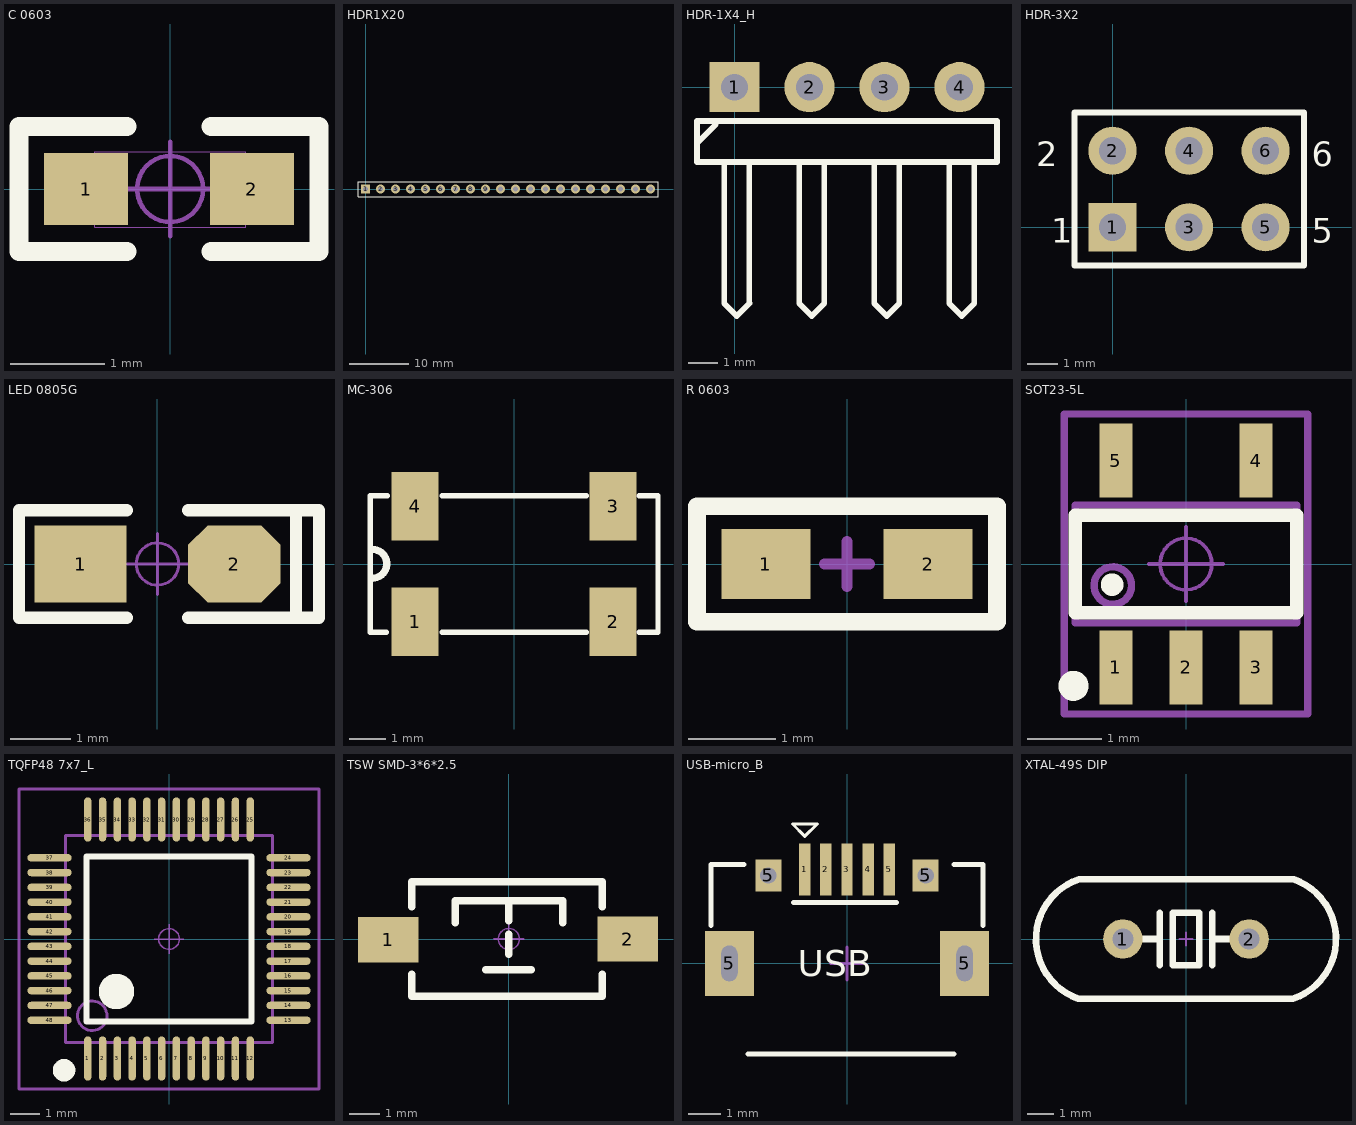
[diagram p0: the footprints below, top view; thin cyan lines are the x and y axes]
# Altium footprint library MISC82227-4.PcbLib: 12 footprints
Each footprint in its own frame and in the unit in brackets; x right, y up, seen from the top. Pads: shape width x height; smd on the part's side, far side on the other; paste and mask are expansions set on the pad; w line width, h text height; cw(c..) or ccw(c..) is an arc to the next point about the centre after c.

## C 0603 [mil] "Non-polarised SMD capacitor"
pads (2):
  rect 35x30 smd: 1(-35,0) 2(34,0)
Top Overlay:
  lines w8: -18,-26 -63,-26 -63,26 -18,26 ; 17,-26 62,-26 62,26 17,26
Mechanical 13:
  lines w0.39: -31.5,-16 31.5,-16 31.5,15.5 -31.5,15.5 -31.5,-16
Mechanical 15:
  circle w1.97: c0,0 r13.78
  lines w1.97: -19.68,0 19.68,0 ; 0,-19.68 0,19.68
3D body "C 0603.STEP": height 31.89, standoff -0.39, extent -31.5,-16.14 31.5,16.14

## HDR1X20 [mm] "Connector; Header; 20 Position"
height 4.32
pads (20):
  rect 1.5x1.5 hole 0.9: 1(0,0)
  round 1.5 hole 0.9: 2(2.54,0) 3(5.08,0) 4(7.62,0) 5(10.16,0) 6(12.7,0) 7(15.24,0) 8(17.78,0) 9(20.32,0) 10(22.86,0) 11(25.4,0) 12(27.94,0) 13(30.48,0) 14(33.02,0) 15(35.56,0) 16(38.1,0) 17(40.64,0) 18(43.18,0) 19(45.72,0) 20(48.26,0)
Top Overlay:
  lines w0.2: -1.27,-1.27 49.53,-1.27 49.53,1.27 0.635,1.27 -1.27,1.27 -1.27,-1.27

## HDR-1X4_H [mm] "Right-angle pin header, 4 pins"
pads (4):
  rect 1.7x1.7 hole 0.9: 1(0,0)
  round 1.7 hole 0.9: 2(2.54,0) 3(5.08,0) 4(7.62,0)
Top Overlay:
  lines w0.2: -1.27,-1.905 -0.635,-1.27 ; -0.348,-2.54 -0.348,-7.332 0.075,-7.755 0.499,-7.332 0.508,-7.323 ; 0.499,-7.323 0.499,-2.54 ; 2.192,-2.54 2.192,-7.332 2.615,-7.755 3.039,-7.332 ; 3.039,-7.323 3.039,-2.54 ; 4.732,-2.54 4.732,-7.332 5.155,-7.755 5.579,-7.332 ; 5.579,-7.323 5.579,-2.54 ; 7.272,-2.54 7.272,-7.332 7.695,-7.755 8.119,-7.332 ; 8.119,-7.323 8.119,-2.54 ; -1.27,-2.54 8.89,-2.54 8.89,-1.143 0.508,-1.143 -1.27,-1.143 -1.27,-2.54
3D body "HDR2.54-1P_H.STEP": height 4.85, standoff -3, extent 6.35,-7.77 8.89,1.27
3D body "HDR2.54-1P_H.STEP": height 4.85, standoff -3, extent 3.81,-7.77 6.35,1.27
3D body "HDR2.54-1P_H.STEP": height 4.85, standoff -3, extent 1.27,-7.77 3.81,1.27
3D body "HDR2.54-1P_H.STEP": height 4.85, standoff -3, extent -1.27,-7.77 1.27,1.27

## HDR-3X2 [mm] "Dual-row pin header, 3x2 pins"
pads (6):
  rect 1.6x1.6 hole 0.9: 1(0,0)
  round 1.6 hole 0.9: 2(0,2.54) 3(2.54,0) 4(2.54,2.54) 5(5.08,0) 6(5.08,2.54)
Top Overlay:
  lines w0.2: 1.482,-1.27 6.35,-1.27 ; 6.35,-1.27 6.35,3.81 -1.27,3.81 -1.27,-1.27 6.35,-1.27
  text "6" at 6.604,2.032 h0.81
  text "5" at 6.604,-0.508 h0.81
  text "2" at -2.54,2.032 h0.81
  text "1" at -2.032,-0.508 h0.81
3D body "HDR2.54-1x2P.STEP": height 8.5, standoff -3, extent 3.81,-1.27 6.35,3.81
3D body "HDR2.54-1x2P.STEP": height 8.5, standoff -3, extent -1.27,-1.27 1.27,3.81
3D body "HDR2.54-1x2P.STEP": height 8.5, standoff -3, extent 1.27,-1.27 3.81,3.81

## LED 0805G [mil] "Green 0805LED"
pads (2):
  rect 60x50 smd: 1(-50,0)
  oct 60x50 smd: 2(50,0)
Top Overlay:
  lines w8: -20,-35 -90,-35 -90,35 -20,35 ; 20,-35 105,-35 105,35 20,35 ; 90,-35 90,35
Mechanical 15:
  circle w1.97: c0,0 r13.78
  lines w1.97: -19.68,0 19.68,0 ; 0,-19.68 0,19.68
3D body "LED 0805玻璃罩.STEP": height 31.69, standoff 12.01, extent -29.49,-24.65 29.49,24.65
3D body "LED 0805-G.STEP": height 26.33, standoff -0.16, extent -39.37,-24.65 39.37,24.65

## MC-306 [mm]
height 1.6
pads (4):
  rect 1.3x1.9 smd: 1(-2.75,-1.6) 2(2.75,-1.6) 3(2.75,1.6) 4(-2.75,1.6)
Top Overlay:
  lines w0.152: -3.556,-1.9 -4,-1.9 -4,1.9 -3.531,1.9 ; -2,-1.9 2,-1.9 ; -2,1.9 2,1.9 ; 3.48,-1.9 4,-1.9 4,1.9 3.48,1.9
  lines w0.2: -3.937,-0.394 ccw(c-3.937,0.006) -3.937,0.406

## R 0603 [mil] "1/10W SMD resistor"
pads (2):
  rect 40x31.5 smd: 1(-36.5,0) 2(36.5,0)
Top Overlay:
  lines w8: -67.5,-26 -67.5,26 67.5,26 67.5,-26 -67.5,-26
Mechanical 15:
  lines w5: -10,0 10,0 ; 0,-10 0,10
3D body "R 0603.STEP": height 15.79, standoff -0.13, extent -31.5,-15.75 31.5,15.75

## SOT23-5L [mm] "3x1.6x1.1mm (LxWxH)"
pads (5):
  rect 0.45x1 smd: 1(-0.95,-1.4) 2(0,-1.4) 3(0.95,-1.4) 4(0.95,1.4) 5(-0.95,1.4)
Top Overlay:
  circle w0.254: c-1.524,-1.651 r0.076
  circle w0.254: c-1.001,-0.279 r0.025
  lines w0.178: -1.5,-0.66 -1.5,0.66 1.5,0.66 1.5,-0.66 -1.5,-0.66
Mechanical 13:
  circle w0.1: c-0.992,-0.292 r0.254
  lines w0.1: -1.5,-0.8 1.5,-0.8 1.5,0.8 -1.5,0.8 -1.5,-0.8
Mechanical 15:
  circle w0.05: c0,0 r0.35
  lines w0.05: -0.5,0 0.5,0 ; 0,-0.5 0,0.5
  lines w0.1: -1.651,-2.032 1.651,-2.032 1.651,2.032 -1.651,2.032 -1.651,-2.032
3D body "SOT23-5.STEP": height 1.15, standoff -0.03, extent -1.5,-1.403 1.5,1.403

## TQFP48 7x7_L [mm] "48 pins, body: 7x7mm, pitch: 0.5mm"
height 1.6
pads (48):
  oval 0.25x1.5 smd: 1(-2.75,-4.046) 2(-2.25,-4.046) 3(-1.75,-4.046) 4(-1.25,-4.046) 5(-0.75,-4.046) 6(-0.25,-4.046) 7(0.25,-4.046) 8(0.75,-4.046) 9(1.25,-4.046) 10(1.75,-4.046) 11(2.25,-4.046) 12(2.75,-4.046) 25(2.75,4.046) 26(2.25,4.046) 27(1.75,4.046) 28(1.25,4.046) 29(0.75,4.046) 30(0.25,4.046) 31(-0.25,4.046) 32(-0.75,4.046) 33(-1.25,4.046) 34(-1.75,4.046) 35(-2.25,4.046) 36(-2.75,4.046)
  oval 1.5x0.25 smd: 13(4.046,-2.75) 14(4.046,-2.25) 15(4.046,-1.75) 16(4.046,-1.25) 17(4.046,-0.75) 18(4.046,-0.25) 19(4.046,0.25) 20(4.046,0.75) 21(4.046,1.25) 22(4.046,1.75) 23(4.046,2.25) 24(4.046,2.75) 37(-4.046,2.75) 38(-4.046,2.25) 39(-4.046,1.75) 40(-4.046,1.25) 41(-4.046,0.75) 42(-4.046,0.25) 43(-4.046,-0.25) 44(-4.046,-0.75) 45(-4.046,-1.25) 46(-4.046,-1.75) 47(-4.046,-2.25) 48(-4.046,-2.75)
Top Overlay:
  circle w0.6: c-1.778,-1.778 r0.3
  circle w0.508: c-3.556,-4.445 r0.127
  lines w0.2: -2.794,-2.794 2.794,-2.794 2.794,2.794 -2.794,2.794 -2.794,-2.794
Mechanical 13:
  circle w0.1: c-2.6,-2.6 r0.5
  lines w0.1: -3.5,-3.5 3.5,-3.5 3.5,3.5 -3.5,3.5 -3.5,-3.5
Mechanical 15:
  circle w0.05: c0,0 r0.35
  lines w0.05: -0.5,0 0.5,0 ; 0,-0.5 0,0.5
  lines w0.1: -5.08,-5.08 5.08,-5.08 5.08,5.08 -5.08,5.08 -5.08,-5.08
3D body "TQFP48 7x7.STEP": height 1.05, standoff 0, extent -4.502,-4.502 4.502,4.502

## TSW SMD-3*6*2.5 [mm] "3*6*2.5mm"
pads (2):
  rect 2x1.5 smd: 1(-3.996,-0.02) 2(3.937,0)
Top Overlay:
  lines w0.254: -3.212,-1.168 -3.212,-1.9 3.088,-1.9 3.088,-1.168 ; -3.212,1.067 -3.212,1.9 3.088,1.9 3.088,1.067 ; -1.778,0.533 -1.778,1.27 1.778,1.27 1.778,0.533 ; -0.762,-1.016 0.737,-1.016 ; 0,-0.508 0,0.152 ; 0,0.61 0,1.27
Mechanical 15:
  circle w0.05: c0,0 r0.35
  lines w0.05: -0.5,0 0.5,0 ; 0,-0.5 0,0.5
3D body "TSW SMD-3x6x2.5.STEP": height 2.59, standoff -0.03, extent -4,-1.877 4,1.623

## USB-micro_B [mm] "Micro USB, 5.7*7.8*2.5mm"
pads (9):
  rect 0.35x1.6 smd: 1(-1.3,2.9) 2(-0.65,2.9) 3(0,2.9) 4(0.65,2.9) 5(1.3,2.9)
  rect 1.5x2 hole 0.5 slot 1.1 at 90 deg: 5(-3.625,0) 5(3.625,0)
  rect 0.8x1 hole 0.5: 5(-2.425,2.71) 5(2.425,2.71)
Top Overlay:
  lines w0.1: -1.681,4.297 -1.3,3.916 -0.919,4.297 -1.681,4.297
  lines w0.152: -4.191,1.168 -4.191,3.048 -3.175,3.048 ; -3.048,-2.794 3.302,-2.794 ; -1.65,1.875 1.525,1.875 ; 3.302,3.048 4.191,3.048 4.191,1.168
  text "USB" at -1.524,-0.402 h0.81
Mechanical 15:
  lines w0.1: -0.508,0 0.508,0 ; 0,-0.508 0,0.508
3D body "USB micro_A.STEP": height 2.8, standoff -0.95, extent -4.001,-2.71 4.001,2.89

## XTAL-49S DIP [mm]
pads (2):
  round 1.5 hole 0.8: 1(-2.4,0) 2(2.4,0)
Top Overlay:
  lines w0.254: -4.09,-2.275 4.059,-2.275 ccw(c3.298,0.003) 4.09,2.271 ; -4.09,-2.271 cw(c-3.298,-0.003) -4.059,2.275 4.09,2.275 ; -1.6,0 -1,0 ; -1,-1 -1,1 ; 1,-1 1,1 ; 1,0 1.6,0 ; -0.5,-1 -0.5,1 0.5,1 0.5,-1 -0.5,-1
Mechanical 15:
  lines w0.076: -0.254,0 0.254,0 ; 0,-0.254 0,0.254
3D body "SW3dPS-HP49US.STEP": height 3.5, standoff -4, extent -5.675,-2.35 5.675,2.3